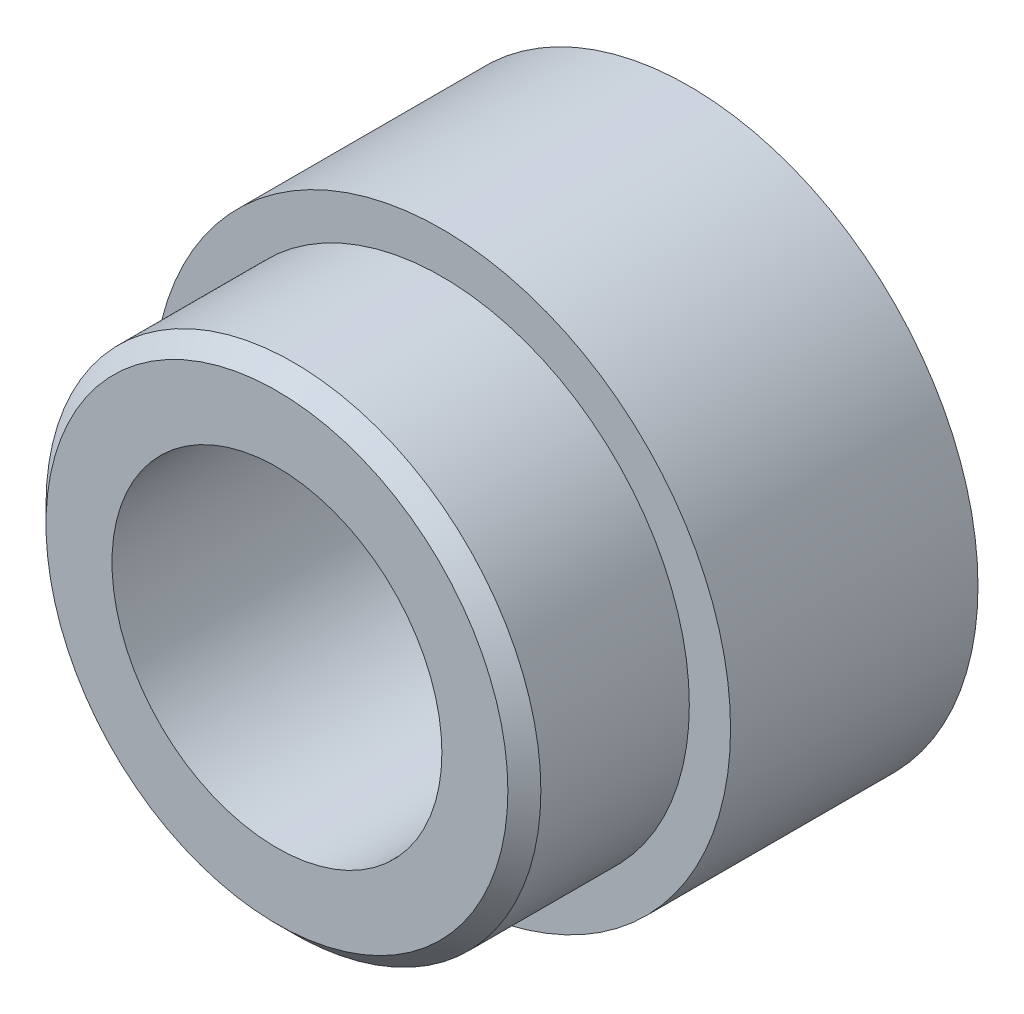
SolidWorks part; units mm, degrees
ref_plane "Front Plane" through (0, 0, 0) normal (0, 0, 1) x (1, 0, 0)
ref_plane "Top Plane" through (0, 0, 0) normal (0, 1, 0) x (1, 0, 0)
ref_plane "Right Plane" through (0, 0, 0) normal (1, 0, 0) x (0, 0, -1)
sketch "Sketch1" plane through (0, 0, 0) normal (0, 0, 1) x (1, 0, 0)
  circle A0 centre (0, 0) radius 17.5
  circle A1 centre (0, 0) radius 10
  dimension "D1" = 35
  dimension "D2" = 20
extrude "Boss-Extrude1" add sketch "Sketch1" along normal blind 25
sketch "Sketch2" plane through (0, 0, 25) normal (0, 0, 1) x (1, 0, 0)
  circle A0 centre (0, 0) radius 17.5
  circle A1 centre (0, 0) radius 15
  dimension "D1" = 30
extrude "Cut-Extrude1" cut sketch "Sketch2" against normal blind 10
chamfer "Chamfer1" distance 1 angle 45 1 edges at (15, 0, 25)
